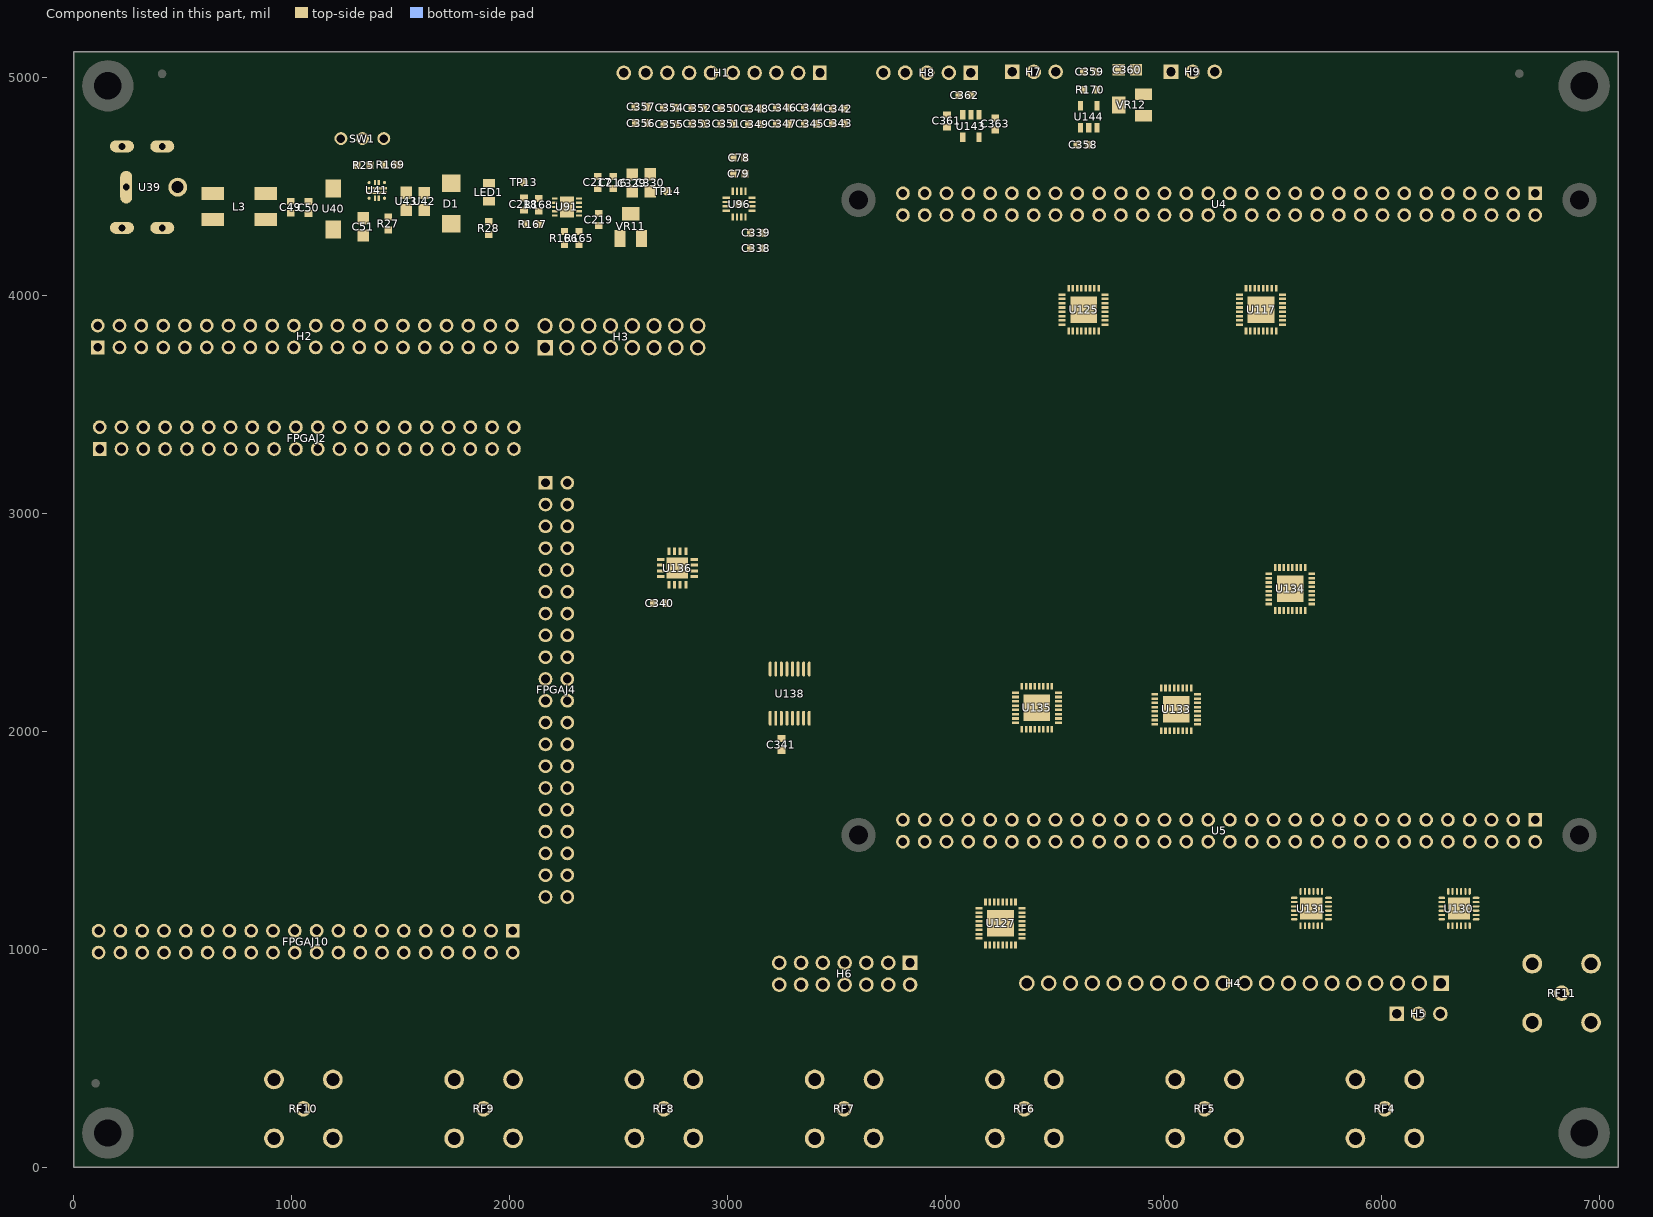
[diagram p0: the components of this part, seen from the top]
# Altium PCB MISC82799.PcbDoc (part 5 of 5)
Units mil, origin at the board's own origin, x right, y up, seen from the top; angles counter-clockwise.
Board outline 7086.61 x 5118.11 mil, 4 copper layers (Top Layer, GND, POWER, Bottom Layer); 95 components, 232 nets, 857 pads, 1291 vias.

## Via types
v1: diameter 20, hole 12, Top Layer to Bottom Layer, 1291 vias

## Nets (pads, with @x,y where several pads share a name; then routed paths per layer and width w, separated by ;. In a path a pad name is that pad's centre, name@x,y a point inside that pad or via, vN(x,y) a via of type N, cw(c..) or ccw(c..) an arc to the next point about the centre after c; other vN are vias at no path point) (continued)
pads on no net: FPGAJ2.2 FPGAJ2.39 FPGAJ2.40 FPGAJ4.2 FPGAJ4.6 FPGAJ4.17 FPGAJ4.18 FPGAJ4.19 FPGAJ4.20 FPGAJ4.21 FPGAJ4.22 FPGAJ4.23 FPGAJ4.24 FPGAJ4.25 FPGAJ4.26 FPGAJ4.27 FPGAJ4.28 FPGAJ4.29 FPGAJ4.30 FPGAJ4.31 FPGAJ4.32 FPGAJ4.33 FPGAJ4.34 FPGAJ4.35 FPGAJ4.36 FPGAJ4.39 FPGAJ4.40 FPGAJ10.2 FPGAJ10.3 FPGAJ10.4 FPGAJ10.5 FPGAJ10.6 FPGAJ10.7 FPGAJ10.8 FPGAJ10.9 FPGAJ10.10 FPGAJ10.11 FPGAJ10.12 FPGAJ10.13 FPGAJ10.14 FPGAJ10.15 FPGAJ10.16 FPGAJ10.17 FPGAJ10.18 FPGAJ10.19 FPGAJ10.20 FPGAJ10.21 FPGAJ10.22 FPGAJ10.23 FPGAJ10.24 FPGAJ10.25 FPGAJ10.26 FPGAJ10.27 FPGAJ10.28 FPGAJ10.29 FPGAJ10.30 FPGAJ10.31 FPGAJ10.32 FPGAJ10.33 FPGAJ10.34 FPGAJ10.35 FPGAJ10.36 FPGAJ10.39 FPGAJ10.40 H1.9 H1.10 H2.37 H2.38 H2.39 H2.40 SW1.1 U41.2 U41.3 U41.4 U41.10 U117.12 U117.13 U117.26 U117.27 U117.28 U117.30 U117.32 U125.11 U125.12 U125.13 U125.26 U125.28 U125.30 U125.32 U127.11 U127.12 U127.13 U127.26 U127.28 U127.30 U127.32 U133.12 U133.13 U133.17 U133.18 U133.19 U133.20 U133.26 U133.27 U133.28 U133.30 U133.32 U134.12 U134.13 U134.26 U134.27 U134.28 U134.30 U134.32 U135.12 U135.13 U135.17 U135.18 U135.19 U135.20 U135.26 U135.27 U135.28 U135.30 U135.32 U136.7 U143.4 VR11.1 VR12.1
copper on no net:
  other v1: 4331,2492 4383,2551

## Polygon pours and split planes (outlines as drawn)
GND on Top Layer "Bottom Layer-No Net" (solid, remove dead copper): -301,4903 -327,4877 -327,-264 7336,-264 7412,-188 7564,-36 7564,369 7564,5245 7412,5397 7272,5537 6867,5537 -60,5537 -238,5359 -301,5296 -301,4910
3P3V on Top Layer "Bottom Layer-No Net" (solid, remove dead copper): 2305,4444 2305,4421 2306,4420 2308,4418 2315,4418 2635,4418 2675,4378 2718,4378 2773,4378 2782,4387 2794,4399 2794,4414 2794,4462 2773,4483 2750,4506 2667,4506 2337,4506 2315,4484 2305,4474 2305,4446
NetC358_2 on Top Layer "Bottom Layer-No Net" (solid, remove dead copper): 4397,4710 4397,4635 4411,4621 4447,4585 4576,4585 4659,4585 4671,4597 4699,4625 4699,4670 4699,4715 4679,4735 4674,4740 4674,4762 4674,4788 4670,4792 4668,4792 4647,4792 4645,4790 4643,4788 4643,4783 4643,4657 4636,4650 4627,4641 4613,4641 4511,4641 4495,4657 4482,4670 4482,4694 4482,4727 4476,4733 4472,4737 4462,4737 4413,4737 4401,4725 4397,4721 4397,4711
5V_NEG on Top Layer "Bottom Layer-No Net" (solid, remove dead copper): 4472,5037 4472,4893 4497,4868 4519,4846 4593,4846 4628,4846 4633,4851 4651,4869 4651,4925 4651,5050 4645,5056 4630,5071 4585,5071 4493,5071 4480,5058 4472,5050 4472,5039
NetC363_2 on Top Layer "Bottom Layer-No Net" (solid, remove dead copper): 4141,4843 4141,4806 4142,4805 4149,4798 4215,4798 4336,4798 4392,4854 4446,4908 4446,4995 4446,5048 4438,5056 4433,5061 4410,5061 4383,5061 4379,5057 4367,5045 4367,5014 4367,4932 4348,4913 4322,4887 4248,4887 4170,4887 4149,4866 4141,4858 4141,4843
5V on Top Layer "Bottom Layer-No Net" (solid, remove dead copper): 4077,5031 4077,5011 4077,4974 4085,4966 4099,4952 4099,4865 4099,4807 4102,4804 4103,4803 4109,4803 4127,4803 4129,4805 4131,4807 4131,4814 4131,4869 4152,4890 4172,4910 4172,4987 4172,5056 4163,5065 4159,5069 4146,5069 4086,5069 4082,5065 4077,5060 4077,5030
5V on Top Layer "Bottom Layer-No Net" (solid, remove dead copper): 1342,4475 1342,4466 1343,4465 1344,4464 1349,4464 1442,4464 1451,4455 1465,4441 1532,4441 1646,4441 1668,4463 1676,4471 1720,4471 1801,4471 1811,4481 1822,4492 1915,4492 2001,4492 2010,4483 2018,4475 2018,4460 2018,4444 2023,4439 2033,4429 2065,4429 2157,4429 2166,4420 2167,4419 2167,4410 2167,4408 2171,4404 2176,4399 2200,4399 2218,4399 2220,4401 2221,4402 2221,4405 2221,4628 2201,4648 2165,4684 2024,4684 1578,4684 1560,4666 1549,4655 1549,4614 1549,4570 1537,4558 1531,4552 1500,4552 1474,4552 1466,4544 1458,4536 1458,4516 1458,4489 1449,4480 1447,4478 1438,4478 1344,4478 1342,4476
NetC49_2 on Top Layer "Bottom Layer-No Net" (solid, remove dead copper): 826,4502 826,4439 832,4433 836,4429 917,4429 943,4429 956,4416 958,4414 998,4414 1118,4414 1132,4428 1146,4442 1148,4444 1300,4444 1317,4444 1325,4452 1328,4455 1328,4465 1328,4471 1332,4475 1339,4482 1349,4482 1440,4482 1441,4483 1441,4486 1441,4497 1440,4498 1439,4499 1433,4499 1336,4499 1320,4515 1318,4517 1318,4575 1318,4619 1317,4620 1312,4625 1290,4625 885,4625 852,4592 826,4566 826,4502
NetL3_2 on Top Layer "Bottom Layer-No Net" (solid, remove dead copper): 166,4686 166,4214 183,4197 200,4180 287,4180 673,4180 688,4195 692,4199 692,4332 692,4377 689,4380 687,4382 679,4382 580,4382 567,4369 548,4350 470,4350 373,4350 352,4371 341,4382 341,4436 341,4600 365,4624 375,4634 411,4634 463,4634 474,4645 482,4653 482,4673 482,4736 477,4741 470,4748 451,4748 186,4748 174,4736 166,4728 166,4686
NetL3_1 on Top Layer "Bottom Layer-No Net" (solid, remove dead copper): 425,4520 425,4494 425,4469 437,4457 461,4433 641,4433 695,4433 700,4438 705,4443 705,4468 705,4562 689,4578 680,4587 596,4587 446,4587 430,4571 425,4566 425,4520
GND on Bottom Layer "Bottom Layer-No Net" (solid, remove dead copper): -428,4574 -428,-36 -99,-365 28,-492 737,-492 7196,-492 7424,-264 7804,116 7804,471 7804,4954 7247,5511 6892,5866 6462,5866 104,5866 -149,5613 -428,5334 -428,4625
3P3V on Bottom Layer "Bottom Layer-No Net" (solid, remove dead copper): 2324,4241 2324,4205 2328,4201 2333,4196 2347,4196 2534,4196 2556,4218 2574,4236 3100,4236 3122,4236 3139,4236 3151,4248 3167,4264 3167,4294 3167,4327 3186,4346 3406,4566 3407,4565 5000,4565 5041,4565 5200,4565 5232,4597 5273,4638 5273,5005 5273,5068 5268,5073 5260,5081 5230,5081 5209,5081 5200,5072 5195,5067 5195,5032 5195,4696 5166,4667 5126,4627 4503,4627 4068,4627 4039,4656 3981,4714 3981,4862 3981,4899 4005,4923 4053,4971 4053,5011 4053,5051 4048,5056 4042,5062 4029,5062 3993,5062 3985,5054 3974,5043 3974,5024 3974,4998 3955,4979 3886,4910 3886,4821 3886,4723 3848,4685 3829,4666 3693,4666 3358,4666 3147,4455 3074,4382 3030,4382 2885,4382 2831,4436 2811,4456 2772,4456 2700,4456 2674,4430 2499,4255 2369,4255 2338,4255 2324,4241
NetC358_2 on Bottom Layer "Bottom Layer-No Net" (solid, remove dead copper): 4262,5029 4262,4806 4401,4667 4411,4657 4456,4657 4468,4657 4471,4660 4479,4668 4479,4679 4479,4729 4392,4816 4345,4863 4345,5017 4345,5057 4336,5066 4332,5070 4315,5070 4274,5070 4268,5064 4262,5058 4262,5029
GND on GND (split plane): 7066.52,20.1 20.1,20.1 20.1,5098.01 7066.52,5098.01
5V on POWER (split plane): 4261.91,4238 4262.26,4235.39 4263.26,4232.96 4264.87,4230.87 4346.87,4148.87 4348.96,4147.26 4351.39,4146.26 4354,4145.91 4613.82,4145.91 4648.91,4110.82 4648.91,4029 4649.26,4026.39 4650.26,4023.96 4651.87,4021.87 4690.87,3982.87 4692.96,3981.27 4694.68,3980.55 4695.39,3980.26 4698,3979.91 4907,3979.91 4909.61,3980.26 4912.04,3981.27 4914.13,3982.87 4956.13,4024.87 4957.74,4026.96 4958.03,4027.67 4958.74,4029.39 4959.09,4032 4959.09,4132.82 5003.18,4176.91 5395.82,4176.91 5436.91,4135.82 5436.91,4011 5437.26,4008.39 5438.26,4005.96 5439.87,4003.87 5829.91,3613.82 5829.91,2708.18 5761.82,2640.09 3609,2640.09 3606.39,2639.74 3603.96,2638.73 3601.87,2637.13 3278.82,2314.09 3157.18,2314.09 2799.13,2672.13 2797.04,2673.73 2794.61,2674.74 2792,2675.09 2693,2675.09 2690.39,2674.74 2688.67,2674.03 2687.96,2673.73 2685.87,2672.13 2612.87,2599.13 2611.26,2597.04 2610.26,2594.61 2609.91,2592 2609.91,2283 2610.26,2280.39 2611.26,2277.96 2612.87,2275.87 3088.87,1799.87 3090.96,1798.27 3093.39,1797.26 3096,1796.91 3847,1796.91 3849.61,1797.26 3852.04,1798.27 3854.13,1799.87 4136.18,2081.91 5462.82,2081.91 5823.87,1720.87 5825.96,1719.27 5827.68,1718.55 5828.39,1718.26 5831,1717.91 6243.82,1717.91 6392.91,1568.82 6392.91,1290.18 6347.82,1245.09 6141.18,1245.09 6090.13,1296.13 6088.04,1297.73 6085.61,1298.74 6083,1299.09 5739,1299.09 5736.39,1298.74 5733.96,1297.73 5731.87,1296.13 5686.82,1251.09 4650,1251.09 4647.39,1250.74 4644.96,1249.73 4642.87,1248.13 4481.82,1087.09 4411,1087.09 4408.39,1086.74 4405.96,1085.73 4403.87,1084.13 4372.87,1053.13 4371.26,1051.04 4370.26,1048.61 4369.91,1046 4369.91,619 4370.26,616.39 4371.26,613.96 4372.87,611.87 4444.87,539.87 4446.96,538.27 4447.67,537.97 4449.39,537.26 4452,536.91 7066.52,536.91 7066.52,20.1 20.1,20.1 20.1,5098.01 4261.91,5098.01
5V_NEG on POWER (split plane): 7066.52,557.09 4456.18,557.09 4390.09,623.18 4390.09,1041.82 4415.18,1066.91 4486,1066.91 4488.61,1067.26 4491.04,1068.27 4493.13,1069.87 4654.18,1230.91 5691,1230.91 5693.61,1231.26 5696.04,1232.27 5698.13,1233.87 5743.18,1278.91 6078.82,1278.91 6129.87,1227.87 6131.96,1226.27 6133.68,1225.55 6134.39,1225.26 6137,1224.91 6352,1224.91 6354.61,1225.26 6357.04,1226.27 6359.13,1227.87 6410.13,1278.87 6411.74,1280.96 6412.74,1283.39 6413.09,1286 6413.09,1573 6412.74,1575.61 6411.74,1578.04 6410.13,1580.13 6255.13,1735.13 6253.04,1736.73 6250.61,1737.74 6248,1738.09 5835.18,1738.09 5474.13,2099.13 5472.04,2100.73 5469.61,2101.74 5467,2102.09 4132,2102.09 4129.39,2101.74 4126.96,2100.73 4124.87,2099.13 3842.82,1817.09 3100.18,1817.09 2630.09,2287.18 2630.09,2587.82 2697.18,2654.91 2787.82,2654.91 3145.87,2296.87 3147.96,2295.27 3150.39,2294.26 3153,2293.91 3283,2293.91 3285.61,2294.26 3288.04,2295.27 3290.13,2296.87 3613.18,2619.91 5766,2619.91 5768.61,2620.26 5771.04,2621.27 5773.13,2622.87 5847.13,2696.87 5848.74,2698.96 5849.74,2701.39 5850.09,2704 5850.09,3618 5849.74,3620.61 5849.45,3621.32 5848.74,3623.04 5847.13,3625.13 5457.09,4015.18 5457.09,4140 5456.74,4142.61 5455.74,4145.04 5454.13,4147.13 5407.13,4194.13 5405.04,4195.74 5402.61,4196.74 5400,4197.09 4999,4197.09 4996.39,4196.74 4995.17,4196.24 4993.96,4195.74 4991.87,4194.13 4941.87,4144.13 4940.26,4142.04 4939.26,4139.61 4938.91,4137 4938.91,4036.18 4902.82,4000.09 4702.18,4000.09 4669.09,4033.18 4669.09,4115 4668.74,4117.61 4668.03,4119.33 4667.74,4120.04 4666.13,4122.13 4625.13,4163.13 4623.04,4164.74 4620.61,4165.74 4618,4166.09 4358.18,4166.09 4282.09,4242.18 4282.09,5098.01 7066.52,5098.01

## Keep-outs
Keep-Out Layer:
  the board outline again, w10

## Other copper
POWER (plane layer: these items are gaps in the copper):
  lines w20: 4272,5114 4272,4238 4354,4156 4618,4156 4659,4115 4659,4029 4698,3990 4907,3990 4949,4032 4949,4137 4999,4187 5400,4187 5447,4140 5447,4011 5840,3618 5840,2704 5766,2630 3609,2630 3283,2304 3153,2304 2792,2665 2693,2665 2620,2592 2620,2283 3096,1807 3847,1807 4132,2092 5467,2092 5831,1728 6248,1728 6403,1573 6403,1286 6352,1235 6137,1235 6083,1289 5739,1289 5691,1241 4650,1241 4486,1077 4411,1077 4380,1046 4380,619 4452,547 7080,547

## Silkscreen, mask and mechanical layers (free items; w line width, h text height)
Top Overlay:
  lines w10: 3482.69,1406 7026,1406 7026,4555.61 3482.69,4555.61 3482.69,1406
  text "GND" at 4982,5081 h50
  text "EN" at 5108,5081 h50
  text "3V3" at 5200,5081 h50
  text "D4" at 2994,5079 h50
  text "D2" at 3196,5079 h50
  text "GND" at 3661,5079 h50
  text "5V" at 4095,5079 h50
  text "NC" at 2496,5078 h50
  text "NC" at 2596,5078 h50
  text "D7" at 2696,5078 h50
  text "D6" at 2801,5078 h50
  text "D5" at 2900,5078 h50
  text "D3" at 3098,5078 h50
  text "D1" at 3296,5078 h50
  text "GND" at 3767,5078 h50
  text "GND" at 3872,5078 h50
  text "3V3" at 3983,5078 h50
  text "D0" at 3398,5077 h50
  text "POWER" at 138,4756 h60
  text "S_A2_LEFT" at 1125,3946 h50 r90
  text "S_A0_LEFT" at 1220,3942 h50 r90
  text "GATE_SDO" at 628,3941 h50 r90
  text "DRAIN_SYNC" at 328,3939 h50 r90
  text "GD_A1_LEFT" at 924,3939 h50 r90
  text "NC" at 2021,3939 h50 r90
  text "DRAIN_SDO" at 421,3938 h50 r90
  text "WELL_A3_L" at 1334,3938 h50 r90
  text "GATE_SYNC" at 529,3937 h50 r90
  text "GD_EN_LEFT" at 1029,3937 h50 r90
  text "GD_EN_B" at 726,3936 h50 r90
  text "GD_A2_LEFT" at 822,3936 h50 r90
  text "GND" at 1813,3936 h50 r90
  text "GD_A2_RIGHT" at 228,3935 h50 r90
  text "S_A2_RIGHT" at 1529,3935 h50 r90
  text "NC" at 1930,3935 h50 r90
  text "GD_A0_RIGHT" at 129,3934 h50 r90
  text "S_A0_RIGHT" at 1426,3932 h50 r90
  text "W_EN_LEFT" at 1626,3931 h50 r90
  text "GND" at 2179,3930 h50 r90
  text "W_A1_LEFT" at 1730,3929 h50 r90
  text "DNW_A1" at 2584,3922 h50 r90
  text "DAC_SDI" at 2781,3922 h50 r90
  text "DAC_REF" at 2875,3922 h50 r90
  text "W_A0_R" at 2274,3921 h50 r90
  text "W_A2_R" at 2384,3921 h50 r90
  text "DNW_EN" at 2481,3921 h50 r90
  text "DAC_CS" at 2680,3921 h50 r90
  text "GND" at 2183,3585 h50 r90
  text "SCLK" at 2782,3569 h50 r90
  text "NC" at 1929,3562 h50 r90
  text "NC" at 2022,3562 h50 r90
  text "GND" at 1821,3542 h50 r90
  text "W_A2_L" at 1328,3502 h50 r90
  text "S_A3_R" at 1623,3498 h50 r90
  text "GD_A0_L" at 927,3494 h50 r90
  text "S_EN_R" at 1422,3493 h50 r90
  text "S_A1_R" at 1520,3493 h50 r90
  text "D_RESET" at 429,3489 h50 r90
  text "A1_RIGHT" at 224,3486 h50 r90
  text "G_RESET" at 632,3486 h50 r90
  text "GD_EN_R" at 124,3485 h50 r90
  text "GD_A0_B" at 726,3484 h50 r90
  text "GD_A1_B" at 827,3481 h50 r90
  text "GATE_DIN" at 531,3478 h50 r90
  text "DAC_SDO" at 2881,3478 h50 r90
  text "DRAIN_DIN" at 329,3466 h50 r90
  text "S_A3_LEFT" at 1031,3457 h50 r90
  text "S_A1_LEFT" at 1129,3454 h50 r90
  text "S_EN_LEFT" at 1228,3453 h50 r90
  text "WELL_A0_L" at 1725,3447 h50 r90
  text "W_A3_RIGHT" at 2484,3409 h50 r90
  text "W_A1_RIGHT" at 2386,3408 h50 r90
  text "W_EN_RIGHT" at 2280,3406 h50 r90
  text "CTRL_DNW_A0" at 2581,3364 h50 r90
  text "CTRL_DNW_A2" at 2682,3364 h50 r90
  text "DNW_MUX" at 3247,1018 h50 r90
  text "WELL_RIGHT" at 3349,1011 h50 r90
  text "WELL_LEFT" at 3454,1009 h50 r90
  text "SOURCE_RIGHT" at 3549,1008 h50 r90
  text "SOURCE_LEFT" at 3656,1006 h50 r90
  text "DRAIN_BOTTOM" at 3750,1006 h50 r90
  text "DRAIN_RIGHT" at 3848,1003 h50 r90
  text "GATE_6" at 6088,917 h50 r90
  text "GATE_8" at 6285,912 h50 r90
  text "GATE_7" at 6190,910 h50 r90
  text "GATE_3" at 5789,611 h50 r90
  text "GATE_5" at 5988,609 h50 r90
  text "GATE_2" at 5688,607 h50 r90
  text "GATE_4" at 5887,607 h50 r90
  text "GATE_1" at 5591,602 h50 r90
  text "DRAIN_1" at 4789,594 h50 r90
  text "DRAIN_3" at 4991,593 h50 r90
  text "DRAIN_6" at 5287,593 h50 r90
  text "DRAIN_8" at 5490,593 h50 r90
  text "DRAIN_4" at 5085,590 h50 r90
  text "DRAIN_2" at 4890,589 h50 r90
  text "DRAIN_5" at 5190,589 h50 r90
  text "DRAIN_7" at 5390,588 h50 r90
  text "DRAIN_1" at 3645,582 h50 r90
  text "SOURCE" at 3448,578 h50 r90
  text "DRAIN_2" at 3544,576 h50 r90
  text "BNC_DNW" at 3247,534 h50 r90
  text "PSUB" at 6087,523 h50 r90
  text "BNC_WELL" at 3342,521 h50 r90
  text "GATE_LEFT" at 4488,521 h50 r90
  text "PSUB" at 6188,518 h50 r90
  text "DRAIN_LEFT" at 4387,509 h50 r90
  text "BNC_PSUB" at 6682,505 h60
  text "GATE_RIGHT" at 4690,500 h50 r90
  text "BNC_GATE_2" at 3759,484 h50 r90
  text "BNC_GATE_1" at 3865,484 h50 r90
  text "GATE_BOTTOM" at 4586,443 h50 r90
  text "BNC_PSUB" at 6290,396 h50 r90
  text "BNC_DNW" at 786,136 h60 r90
  text "BNC_WELL" at 1621,119 h60 r90
  text "BNC_SOURCE" at 2436,98 h60 r90
  text "BNC_GATE_1" at 5739,97 h60 r90
  text "BNC_GATE_2" at 4917,89 h60 r90
  text "BNC_DRAIN_1" at 4090,80 h60 r90
  text "BNC_DRAIN_2" at 3256,74 h60 r90